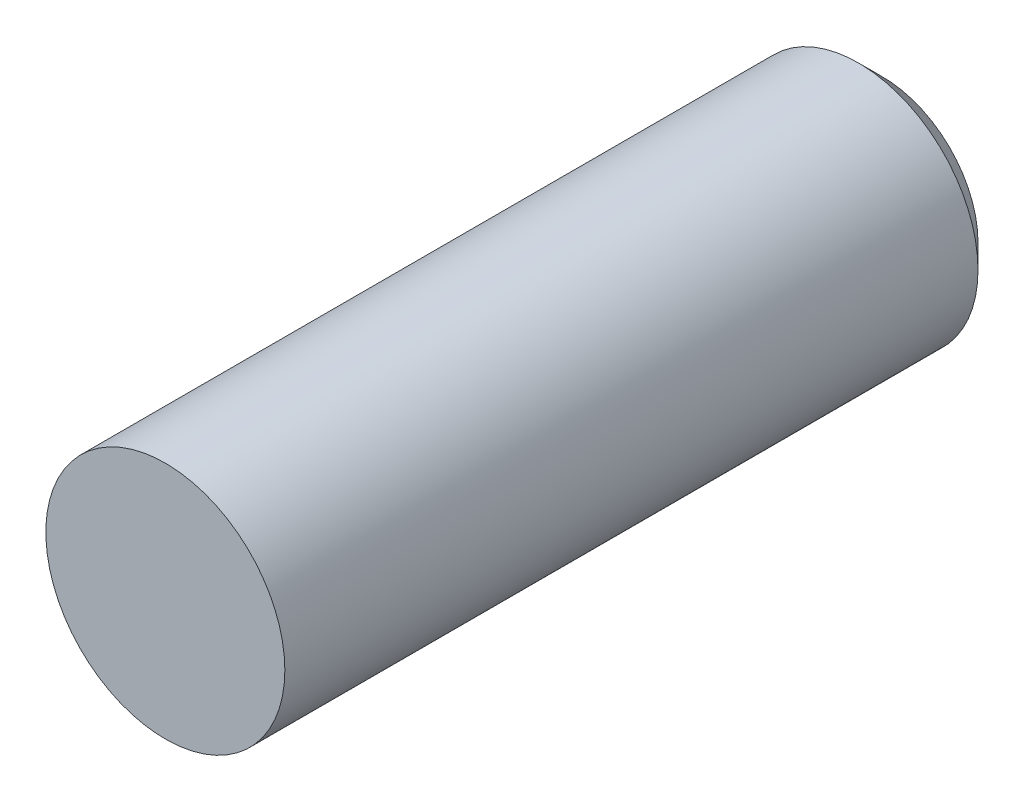
from build123d import *

# Parameters (mm, degrees)
SKETCH1_R           = 5
BOSS_EXTRUDE1_DEPTH = 30
CHAMFER1_SIZE       = 1


with BuildPart() as part:
    # Sketch1 → Boss-Extrude1 (new body)
    with BuildSketch(Plane.XY):
        Circle(SKETCH1_R)
    extrude(amount=BOSS_EXTRUDE1_DEPTH)

    # Chamfer1
    chamfer1_edges = [part.edges().sort_by_distance(p)[0] for p in [
        (-5, 0, 0),
    ]]
    chamfer(chamfer1_edges, length=CHAMFER1_SIZE)


solid = part.part
